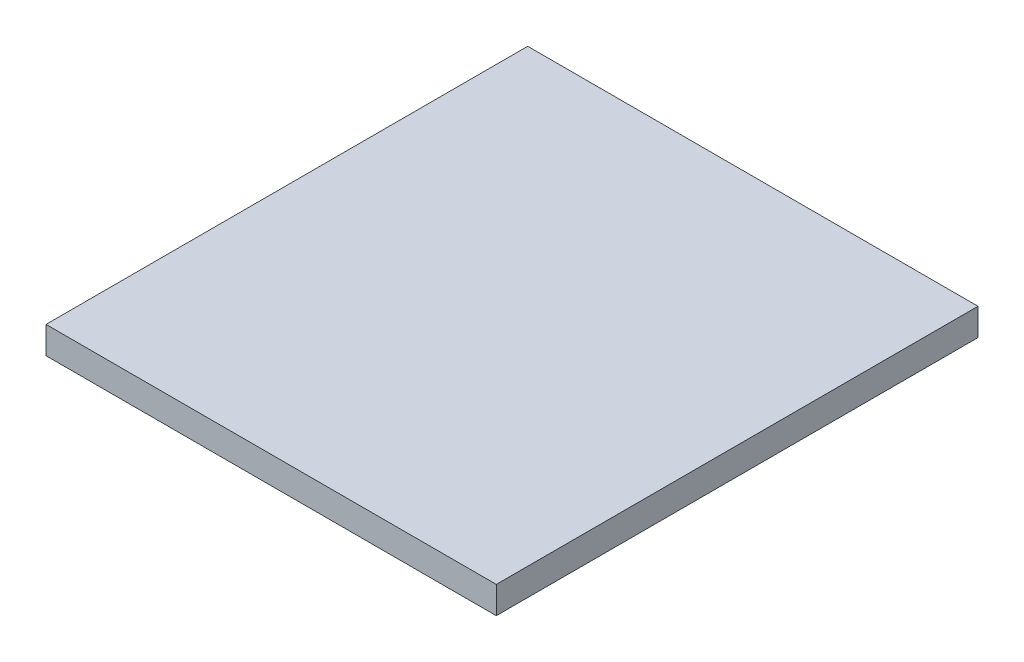
from build123d import *

# Parameters (mm, degrees)
SKETCH1_W           = 31.52
SKETCH1_H           = 33.72
BOSS_EXTRUDE1_DEPTH = 1.9
SCALE1_SCALE        = 0.5


with BuildPart() as part:
    # Sketch1 → Boss-Extrude1 (new body)
    with BuildSketch(Plane(origin=(0, 0, 0), x_dir=(1, 0, 0), z_dir=(0, 1, 0))):
        Rectangle(SKETCH1_W, SKETCH1_H)
    extrude(amount=BOSS_EXTRUDE1_DEPTH)


with BuildPart() as part_1:
    # Scale1: scaled about (0, 0.95, 0)
    add(part.part.scale(SCALE1_SCALE).moved(Location((0, 0.475, 0))))


solid = part_1.part
